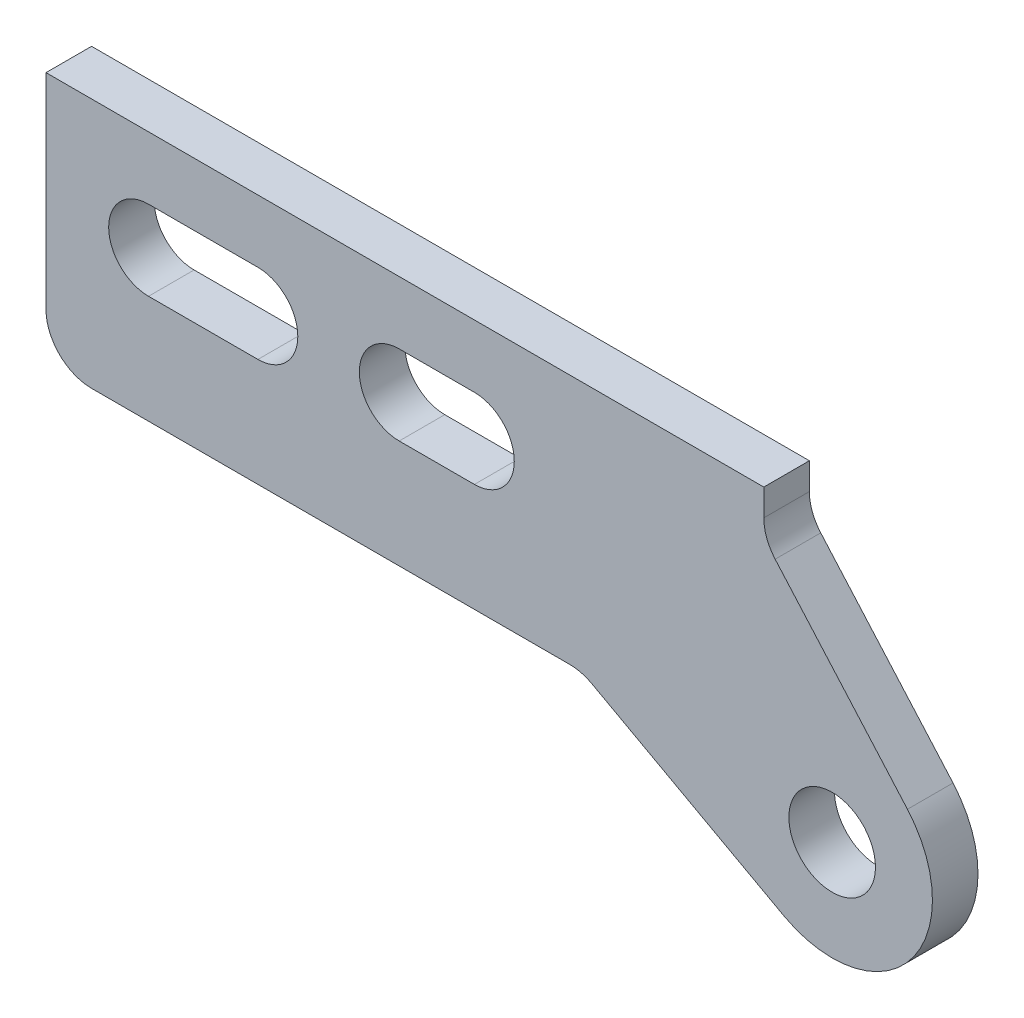
SolidWorks part; units mm, degrees
material "1023 碳钢板 (SS)"
ref_plane "前视基准面" through (0, 0, 0) normal (0, 0, 1) x (1, 0, 0)
ref_plane "上视基准面" through (0, 0, 0) normal (0, 1, 0) x (1, 0, 0)
ref_plane "右视基准面" through (0, 0, 0) normal (1, 0, 0) x (0, 0, -1)
sketch "草图3" plane through (0, 0, 0) normal (0, 0, 1) x (1, 0, 0)
  line L0 (0, 0) -> (-315, 0)
  line L1 (-315, 0) -> (-315, -90)
  line L2 (-295, -110) -> (-85.1109, -110)
  line L3 (0, 0) -> (0, -11.7177)
  line L4 (-75.5157, -112.452) -> (8.8904, -158.6055)
  line L5 (4.9816, -24.9256) -> (63.0404, -90.9426)
  line L6 (-270, -45) -> (-222, -45) construction
  line L7 (-270, -27.5) -> (-222, -27.5)
  line L8 (-270, -62.5) -> (-222, -62.5)
  line L9 (-160, -45) -> (-127, -45) construction
  line L10 (-160, -27.5) -> (-127, -27.5)
  line L11 (-160, -62.5) -> (-127, -62.5)
  arc A1 (8.8904, -158.6055) -> (63.0404, -90.9426) centre (30, -120) ccw
  arc A2 (0, -11.7177) -> (4.9816, -24.9256) centre (20, -11.7177) ccw
  arc A3 (-85.1109, -110) -> (-75.5157, -112.452) centre (-85.1109, -130) cw
  circle A4 centre (30, -120) radius 19
  arc A5 (-315, -90) -> (-295, -110) centre (-295, -90) ccw
  arc A6 (-270, -27.5) -> (-270, -62.5) centre (-270, -45) ccw
  arc A7 (-222, -62.5) -> (-222, -27.5) centre (-222, -45) ccw
  arc A8 (-160, -27.5) -> (-160, -62.5) centre (-160, -45) ccw
  arc A9 (-127, -62.5) -> (-127, -27.5) centre (-127, -45) ccw
  point P14 (-80, -110)
  point P17 (-315, -110)
  point P20 (-246, -45)
  point P25 (-143.5, -45)
  point P32 (0, 0)
  point P33 (-249.6774, -45)
  dimension "D4" = 120
  dimension "D5" = 345
  dimension "D6" = 88
  dimension "D8" = 20
  dimension "D9" = 20
  dimension "D10" = 38
  dimension "D11" = 20
  dimension "D18" = 45
  dimension "D1" = 110
  dimension "D2" = 315
  dimension "D3" = 235
  dimension "D7" = 20
  dimension "D12" = 35
  dimension "D13" = 45
  dimension "D14" = 33
  dimension "D15" = 48
  dimension "D16" = 35
  dimension "D17" = 62
extrude "凸台-拉伸2" add sketch "草图3" along normal blind 20
